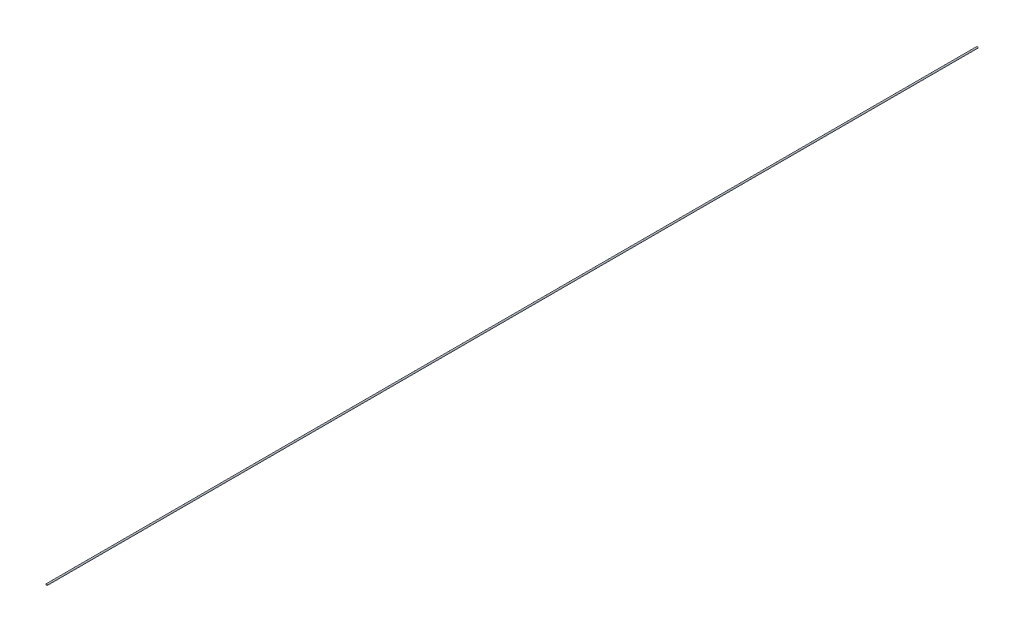
SolidWorks part; units mm, degrees
ref_plane "Front Plane" through (0, 0, 0) normal (0, 0, 1) x (1, 0, 0)
ref_plane "Top Plane" through (0, 0, 0) normal (0, 1, 0) x (1, 0, 0)
ref_plane "Right Plane" through (0, 0, 0) normal (1, 0, 0) x (0, 0, -1)
sketch "Sketch1" plane through (0, 0, 0) normal (0, 0, 1) x (1, 0, 0)
  circle A0 centre (0, 0) radius 1.5
  circle A1 centre (0, 0.95) radius 0.15
  circle A2 centre (0.8227, -0.475) radius 0.15
  circle A3 centre (-0.8227, -0.475) radius 0.15
  point P11 (0, 0)
  dimension "D1" = 3
  dimension "D2" = 0.3
  dimension "D3" = 0.95
  dimension "D4" = 3
extrude "Boss-Extrude1" add sketch "Sketch1" along normal blind 1900
